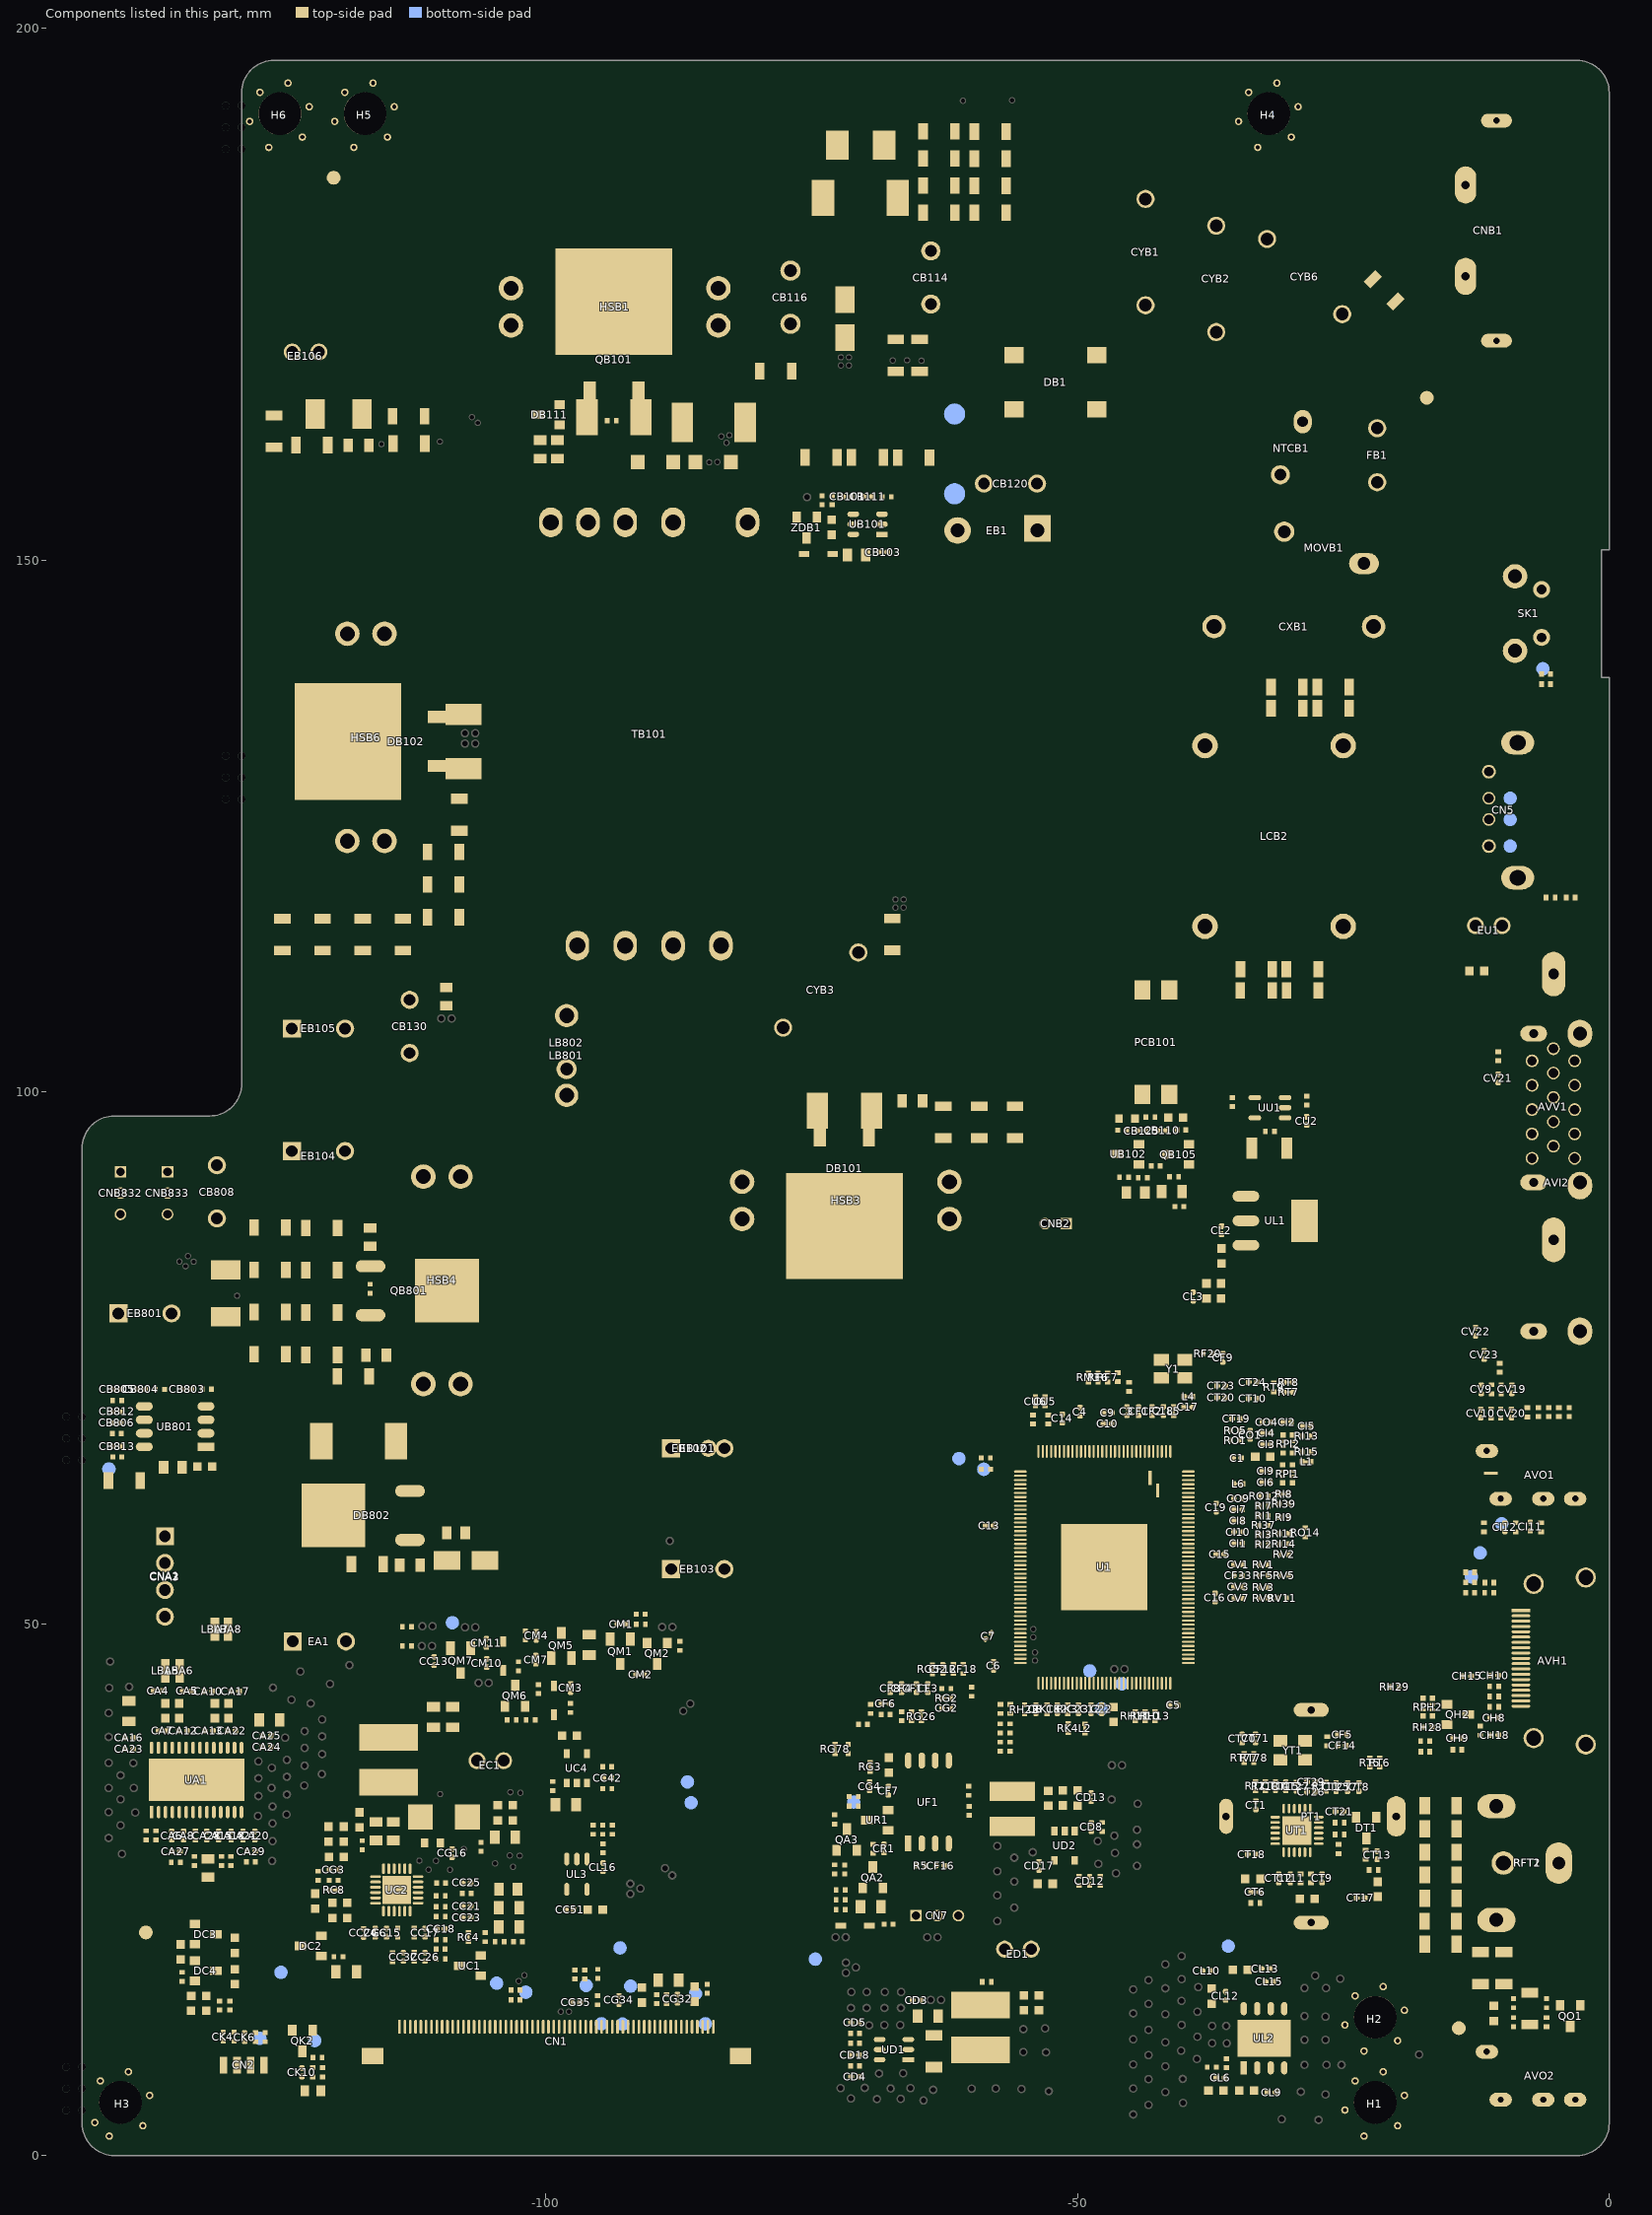
[diagram p0: the components of this part, seen from the top]
# Altium PCB MISC86383-9.PcbDoc (part 6 of 18)
Units mm, origin at the board's own origin, x right, y up, seen from the top; angles counter-clockwise.
Board outline 143.6 x 197 mm, 2 copper layers (TopLayer, BottomLayer), stack 1.571 mm thick; 743 components, 401 nets, 2996 pads, 1077 vias.
Unrouted connection lines stored in the file: 4.

## Footprints (in the part's own frame and the unit in brackets; to place one, negate y for a bottom-side part, rotate by r counter-clockwise, add the part's x,y. Pads: shape width x height; smd on the part's side, far side on the other; paste and mask are expansions set on the pad) (continued)
TO-252 [mm] "与TO-223兼容；15.12.29"
  oval 1.143x2.794 smd: 1(-2.3,-3.6) 3(2.3,-3.6)
  rect 6x6 smd paste-10: 2(0,3.6)
  rect 4x2.6 on Top Paste: 4(0,1.957)
  TopLayer pour cut-out: 2.3,-1.932 2.3,-5.055 -2.345,-5.055 -2.64,-4.996 -2.891,-4.829 -3.058,-4.579 -3.117,-4.284 -3.117,-4.284 -2.299,-4.284 -2.299,-2.699 -3.124,-2.699 -3.066,-2.406 -2.899,-2.157 -2.65,-1.99 -2.356,-1.932 -2.356,-1.932
  silkscreen extent -3.4,-1.34 3.4,7.01, body extent -3.4,-4.15 3.4,6.05, height 2.5
TO-252-GDS [mm] "SC08440  IRLR024N"
  rect 6x6 smd: D(0,0)
  oval 1.143x2.794 smd: G(-2.3,-7.2) S(2.3,-7.2)
  silkscreen extent -3.4,-5.64 3.4,3.4, body extent -3.4,-7.75 3.4,2.45, height 2.5
TP [mm] "TEST POINT   (不带paste  1.27mm 直径）"
  round 1.27 smd paste-1.27: 1(0,0)
TP-TDT [mm] "电源放电测试点，间隔7.5mm"
  round 2 smd paste-2: 1(-3.75,0) 2(3.75,0)
  silkscreen extent -5.75,-2 5.75,2
TP_BL [mm] "TEST POINT,专用背光测试点"
  round 1.27 smd paste-1.27: 1(0,0)
  silkscreen extent -6.4,-0.97 0.95,0.96
TSOT23-6 [mm] "MP65151DJ[MPS]/MP1470"
  rect 1.1x0.5 smd: 1(-1.35,0.95)
  oval 1.1x0.5 smd: 2(-1.35,0) 3(-1.35,-0.95) 4(1.35,-0.95) 5(1.35,0) 6(1.35,0.95)
  silkscreen extent -1.99,-1.5 0.85,2.51, body extent -0.85,-1.5 0.85,1.5, height 1
USB-HD-30 [mm] "广业，USB-20161027-0011，17.07.27"
  oval 2.4x3.3 on Top Overlay: 0(-6.35,8.11) 0(6.35,8.11)
  round 1.5 on Top Overlay: 0(-3.37,10.81) 3(3.63,10.81)
  round 1.3 hole 0.9: 1(-3.37,10.81) 4(3.63,10.81)
  round 1.4 on Top Overlay: 1(-0.87,10.81) 2(1.13,10.81)
  round 1.2 hole 0.9: 2(-0.87,10.81) 3(1.13,10.81)
  oval 2.2x3.1 / inner oval 2.2x3.1 / far side oval 2.9x3.8 hole 1.5 slot 2.4 at 90 deg: 5(6.35,8.11) 6(-6.35,8.11)
  KeepOutLayer pour cut-out: -3.063,12.516 -3.825,12.38 -4.475,11.958 -4.911,11.318 -5.064,10.559 -5.064,10.559 -4.765,9.743 -4.118,9.161 -3.275,8.95 -3.275,8.95 1.967,8.95 2.407,9.037 2.781,9.287 3.03,9.66 3.118,10.101 3.118,10.101 3.118,11.085 3.009,11.632 2.699,12.097 2.234,12.407 1.686,12.516 1.686,12.516
  silkscreen extent -6.65,-0.06 6.65,12, body extent -7.4,-2 7.4,11.9, height 9.4
VR(13*5)-V-7.5 [mm] "为勤,VARISTOR,17.01.04修改为椭圆孔;160105更新椭圆孔 //0424_2019在顶层加整块白油,(12/9/2019按规格书修改高度，从17.5mm改为15.5mm)"
  oval 2.8x2 hole 1.2 slot 2 at 0 deg: 1(3.75,-1.5)
  round 1.9 hole 1.2: 2(-3.75,1.5)
  round 2.1 on Top Overlay: 2(-3.75,1.5)
  oval 3x2.2 on Top Overlay: 2(3.75,-1.5)
  silkscreen extent -6.65,-2.5 6.44,2.5, body extent -6.5,-2.75 6.5,2.75, height 15.5
XTAL-S-3 [mm] "三星（SQ3D03200D2IBA）晶振"
  rect 1.4x1.1 smd: 1(-1.1,-0.85) 2(1.1,-0.85) 3(1.1,0.85) 4(-1.1,0.85)
  silkscreen extent -2.37,-1.91 1.65,1.3, body extent -1.65,-1.3 1.65,1.3, height 0.8
XTAL-S-10 [mm] "铜陵晶威特；SMD3225"
  rect 1.3x1.1 smd: 1(-1.15,-0.9) 2(1.15,-0.9) 3(1.15,0.9) 4(-1.15,0.9)
  silkscreen extent -1.66,-2.5 1.65,1.3, body extent -1.65,-1.3 1.65,1.31, height 0.8

## Part data
AVH1: library part XXX.XXX.0001809-D, "HDMI jack,HDMI Jack,H,Block up,SMD,51U019S-313HFN-E-R-F,FREEPORT-D"
AVI2: library part XXX.XXX.0003577-DLMI, "RCA jack,RCA Jack,AV3,H,Red、White、Yellow,CH5.5,D14,Seal,DIP,RC075-F03L3BY-L,YUQIU-DLMI"
AVO1 AVO2: library part "耳机端子,Earphone Jack,H,Φ3.6,CH5.5,Black,DIP-DLMI"
AVV1: library part WLHD-051A-DLMI-DB15, "CN-DB15-horizontal-#-#-#"
BB101 BB802: library part 004.004.0001046-D, "Ferrite bead,BEAD,50ohm,3.0×4.0,9A,SMD,TP,SMB-302540-K5B-L1,SOLDIER-D"
BB801: library part 004.004.0000346-D, "Ferrite bead,BEAD,80ohm,0805,4000mA,SMD,TP,UPZ2012D800-4R0TF,Sunlord-D"
C1: library part 2.2uF-0402-X5R-±20%-6.3V-D
C2 C11 CA31 CA32 CC50 CD10 CD14 CD15 CD16 CF10 CG31 CL1 CL4 CL5 CL7 CL8 CL11 CL14 CO77 CU1: library part 10uF-0603-X5R-±20%-6.3V-D
C3 C4 C5 C9 C10 C12 C22 CC51 CO1 CO4 CR1 CT6: library part 1uF-0402-X5R-±20%-6.3V-D
C6 C7 C8 C13 C14 C15 C16 C17 C18 C19 C23 CA23 CA24 CA28 CC13 CF7 CF16 CG2 CG3 CG4 CH8 CH9 CH18 CI3 CI4 CI6 CI9 CK4 CK10 CL2 CL3 CM1 CM2 CM4 CT1 CT9 CT11 CT18 CT20 CT21 CT23 CT25 CT27 CU2: library part 0.1uF-0402-Y5V-+80%-20%-16V-D
CA4 CA5 CA10 CA16 CA17 CA25 CA27 CA29 CB103 CF3 CF4 CF6 CF8 CF11 CF12 CI11 CI12: library part 1000pF-0402-X7R-±10%-50V-D
CA6 CA8 CA20 CA21: library part 0.22uF-0402-X5R-±10%-16V-D
CA7 CA12 CA13 CA22: library part 0.22uF-0402-Y5V-+80%-20%-16V-D
CA15 CA18 CC15 CC17 CC18 CG6 CH15: library part 1uF-0402-X5R-±20%-16V-D
CA36 CC29 CC30 CC43 CM5: library part 10uF-0805-X5R-±20%-16V-D
CB101 CB111 CB803 CB813 CI2 CI5 CO9: library part 100pF-0402-NPO-±5%-50V-D
CB102 CB109 CC5 CC7 CC9 CC10 CC11 CC27 CC31 CC34 CC38 CG14 CG33: library part 0.1uF-0603-X7R-±10%-50V-D, "CAP"
CB110 CB125 CB806: library part 1000pF-0402-X7R-±10%-50V-D, "CAP"
CB113: library part 220PF-0805-NPO-±10%-200V-D, "CAP"
CB114: library part C242G472J20A201(编带/法拉)-DAI, "CAP"
CB115: library part 0.1uF-0805-X7R-±10%-50V-D, "CAP"
CB116: library part 004.003.0001889-DHAI, "Ceramic capacitor,CAP CD,1KV,100pF,±5%,SL,OK,5.0mm,DIP,TP,TDK-DHAI"
CB117: library part 1000pF-0805-NPO-±10%-200V-D, "CAP"
CB118: library part "陶瓷电容,CAP MC,1KV,4700pF,±10%,X7R,1206,SMD,TP,ISND-D"
CB120 CB808: library part 004.003.0001665, "Ceramic capacitor,CAP CD,1KV,4700pF,±20%,Y5U,K,5.0mm,DIP,TP,Walsin-DHAI"
CB130: library part 004.003.0000886, "Ceramic capacitor,CAP CD,1KV,4700pF,±20%,Y5U,P,5.0mm,DIP,TP,TongHao-DHAI"
CB801: library part 1uf-0603-X7R-±10%-25V-D
CB804: library part 4700pF-0402-X7R-±10%-50V-D
CB805: library part 0.1uF-0402-X7R-±10%-16V-D
CB809 CB810: library part 004.003.0001392, "Ceramic capacitor,CAP MC,500V,47pF,±5%,NPO,0805,SMD,TP,WALSIN-D"
CB812: library part 0.033uF-0402-X7R-±10%-16V-D
CC1 CC2 CC8 CC12 CC19: library part 22uF-0805-X5R-±20%-6.3V-D
CC4 CC20 CC33 CG22 CG28: library part 1uF-0603-X5R-±10%-50V-D
CC21: library part 1500pF-0402-X7R-±10%-50V-D, "CAP"
CC23 CC24 CC42 CD13 CD17 CG32 CG34 CG35 CL6 CL9 CL10 CL12 CL13 CL15 CL16 CM3: library part 0.1uF-0402-X5R-±20%-16V-D
CC25 CC26 CC32 CH10: library part 33pF-0402-NPO-±5%-50V-D
CD1: library part 004.003.0000514-D, "Ceramic capacitor,CAP MC,16V,10uF,±10%,X5R,1206,SMD,TP-D"
CD2: library part 004.003.0000386-D, "Ceramic capacitor,CAP MC,16V,10uF,±20%,X5R,0805,SMD,TP-D"
CD3 CD4 CD8 CD18: library part 004.003.0000403-D, "Ceramic capacitor,CAP MC,16V,0.1uF,±20%,X5R,0402,SMD,TP-D"
CD5: library part 004.003.0000558-D, "Ceramic capacitor,CAP MC,50V,470pF,±5%,NPO,0402,SMD,TP-D"
CD7 CD9: library part 004.003.0000394-D, "Ceramic capacitor,CAP MC,10V,10uF,±20%,X5R,0603,SMD,TP-D"
CD12: library part 3300pF-0402-X7R-±10%-50V-D
CF1 CF2: library part 004.003.0000527-D, "Ceramic capacitor,CAP MC,50V,18pF,±5%,NPO,0402,SMD,TP-D"
CF5 CU5 CU6 L1 L2 L4 L5 L6 RC4 RC8 RG2 RG3 RG26 RG52 RG78 RI8 RT7 RT8 RT77 RT78: library part 0ohm-0402-PCB-D, "0ohm-0402-PCB-D"
CF9 CF14 CV9 CV10 CV19 CV20 CV21 CV22 CV23: library part 30pF-0402-NPO-±5%-50V-D
CF33 CI1 CI7 CI8 CI10 CV1 CV3 CV7: library part 0.047uF-0402-X7R-±10%-16V-D
CG16: library part 68pF-0402-NPO-±5%-50V-D
CK2: library part 0.01uF-0402-X7R-±10%-50V-D
CK6: library part 10pF-0402-NPO-±5%-50V-D
CM7 CT12 CT19: library part 0.022uF-0402-X7R-±10%-16V-D
CM10: library part 0.022uF-0402-X7R-±10%-50V-D
CM11: library part 004.003.0000398-D, "Ceramic capacitor,CAP MC,16V,0.22uF,±20%,X5R,0402,SMD,TP-D"
CN1: library part XXX.XXX.0004396-D, "FFC connector,FFC connector,60Pin,D0.5,Bottom,lock,SMD,0.5-22-60PBX-P,XFE-D"
CN2: library part 红外接收三极管,Phototransistor,NPN,6.8×3×3.2mm,SMD,HS75438D,VISHAY-D
CN5: library part PKG-003212/P000071027, "USB jack,USB2.0,H,Single,Block up,DIP,U250FD004S1549BY-DLMI"
CN7: library part 3PIN-2.0-D-H-G-带扣-DHMI
CNA1: library part 4PIN-2.54-D-H-G-DHMI
CNA2: library part XXX.XXX.0001836-DLMI, "Connector socket,connect jack,4PIN,D2.50,L,SNAP,STEP,Fool-proofing,Nature,L=3.0mm,DIP,AMA-DLMI"
CNA3: library part 4PIN-2.54-D-H-G-带扣-B-DHMI
CNB1: library part "连接插座,connect jack,2Pin,D8.6,L,SNAP,Fool-proofing,Black,L=4.0mm,DIP,YQ-DLMI", "AC插座-八字侧出"
CNB2: library part XXX.XXX.0001753, "Connector socket,connect jack,2Pin,D2.0,D,L=2.8mm,DIP,AMA-DHMI"
CNB832: library part XXX.XXX.0001754, "Connector socket,connect jack,3Pin,D2.0,D,L=2.8mm,DIP,AMA-DHMI"
CNB833: library part XXX.XXX.0001725-DLMI, "Connector socket,connect jack,3Pin,D2.0,L,SNAP,STEP,Nature,L=2.8mm,DIP,AMA-DLMI"
CT2 CT5: library part 004.003.0000383-D, "Ceramic capacitor,CAP MC,6.3V,10uF,±20%,X5R,0603,SMD,TP-D"
CT7 CT8: library part 004.003.0000530-D, "Ceramic capacitor,CAP MC,50V,22pF,±5%,NPO,0402,SMD,TP-D"
CT10 CT24 CT70 CT71: library part 56pF-0402-NPO-±5%-50V-D
CT13: library part 1.8pF-0402-NPO-±0.25pF-50V-D
CT14 CT15: library part 8pF-0402-NPO-±5%-50V-D
CT17: library part 120pF-0402-NPO-±5%-50V-D
CT26: library part 330pF-0402-NPO-±5%-50V-D
CT29: library part 6800pF-0402-X7R-±10%-50V-D
CT40: library part 4700pF-1206-X7R-±10%-1000V-D
CT41 CT42 CT43 CT44 CT45 CT46 CT47 CT48: library part 1000pF-1206-X7R-±20%-2000V-D
CXB1: library part "X电容,CAP X2,MP,275VAC,0.47uF,±10%,S,15mm-Mini,PC,DIP,BM-DHMI", "CAP"
CYB1 CYB2 CYB3 CYB6: library part "Y电容,CAP Y1,CD,470pF,400VAC,±20%,KS,10mm,Y5U,DIP,Walsin-DHMI", "Y1 capacitor"
DA1 DM1 DM3: library part 1N4148WS-D
DAS1: library part DOLBY_AS2
DB1: library part 004.005.0000860-D, "Bridge rectifier,DIO BRD,3A,800V,YBS,SMD,YBS3010A,YJ-D"
DB101: library part 004.005.0000140-D, "Rectifier diode,DIO SI D1,10A,150V,TO-263,SMD,MBRB10150CT,GOOD-ARK-D"
DB102: library part 004.005.0000473, "Rectifier diode,DIO FRD D1,10A,400V,TO-263,SMD,MURB1040S,GOOD-ARK-D"
DB104 DB804: library part M7(WEJ)-D, "Diode"
DB106 DB801: library part 004.005.0000432-D, "Rectifier diode,DIO SI S,3A,1000V,SMC,SMD,GS3M,GULF-D"
DB107: library part 004.005.0000138-D, "Rectifier diode,DIO FRD S,3A,600V,SMB,SMD,MURS360BT3G,ON-D"
DB109 DB110: library part "整流二极管,DIO FRD S,1.2A,800V,eSGA,SMD,R12K,GOOD-ARK-D"
DB111: library part LBAV70LT1G(LRC)-D, "Diode"
DB112: library part BAV21WS-D, "Diode"
DB802: library part 004.005.0000494-D, "Schottky diode,DIO SBD D1,10A,150V,TO-252,SMD,MBRD10150CT,GOOD-ARK-D"
DC1: library part SK34A-SMA-F-D
DC2 DC3 DC4: library part BAT54S-D
DH2 DH3 DH6 DH7 DI1 DI2 DI3 DI5 DK1 DK2 DO1 DO2 DO3 DR1 DT2 DT3 DU1 DU2 DU3 DU4 DV1 DV2 DV3 DV4 DV5 DV6 DV7 DV8: library part AVLC18S02003-D
DK6: library part 004.005.0000435, "TVS diode,DIO ESD,0.5pF,25V,0402 DFN,SMD,AZ5325-01F.R7G,Amazing-D"
DK20: library part WEJT61RC-871-红色-D
DT1: library part BAV99-BR-D
EA1: library part 470uF-25V-±20%-10×12-105℃-YE-编带-F=5.0(Elite)-DHAI, "Electrolytic"
EB1: library part 004.003.0000164-DLMI, "Aluminium electrolytic capacitor,CAP AL,400V,120uF,±20%,KM,BK,7.5mm,18×35.5,DIP,CapXon-DLMI"
EB101 EB103: library part 470uF-25V-±20%-10×12.5-105℃-GF-编带-F=5.0(CapXon)-DHAI, "Electrolytic"
EB102: library part 270uF-16V-±20%-8×11-105℃-RP-短脚-F=3.5(Elite)-DHMI, "CAP"
EB104 EB105: library part 100uF-63V-±20%-10×12.5-105℃-GF-编带-F=5.0(CapXon)-DHAI, "Electrolytic"
EB106: library part 10uF-50V-±20%-5×11-105℃-GH-编带-F=2.5(CapXon)-DHAI, "Electrolytic"
EB801: library part 47uF-100V-±20%-10×12-105℃-EV-编带-F=5.0(Elite)-DHAI, "Electrolytic"
EC1: library part 100uF-35V-±20%-6.3×11-105℃-KF-编带-F=2.5(CapXon)-DHAI, "Electrolytic"
ED1 EU1: library part 470uF-10V-±20%-6.3×11-105℃-黑底白字-编带-F=2.5-XF-DHAI, "Electrolytic"
EVA1 EVA2 EVA3 EVA4 EVA5 EVA6: library part 7×7×3mm-C-4305防火泡棉-黑色-DLMI, "EVA"
F2: library part 5R1ohm-0402-±5%-1/16W-D
FB1: library part 004.026.0000010-DHMI, "Slow-blow fuse,FUSE T,P,3.15A,250VAC,8.5×4.0×8mm,DIP,TP,Walter-DHMI"
FU1: library part 004.026.0000039-D, "Self-resetting fuse,FUSE PTC,1.1A,6V,1206,SMD,TP,TLC-D"
GD1 GD2 GD3: library part 7.00×8.35mm-尼龙-白色-WQM-DHMI, "Mylar stud"
GL1 GL2 GL3 GL4 GL5: library part 005.002.0000011, "Silicone,0.2g,general,60,white,SLD-8854W,XY-DHMI"
H1 H2 H3 H4 H5 H6: library part "Location hole-D"
HS1: library part 18.8×13.8×5-本色-THD-HS, "SMD heat sink"
HS2: library part 004.040.0008928-D, "Heat sink,15.0×15.0×5.0mm,AL1060H-24,black,high-emissivity paint,stamped with bend,no press-fit legs,YT-D"
HSB1 HSB3 HSB4 HSB6: library part 004.040.0006600-DHMI, "Heat sink,17.5×14.5×0.5mm,red copper sheet,bright tin plated,natural,four pins,WT-DHMI"
LB801: library part SYDR1212-L003-EDL-DHMI, "I-type inductor"
LB802: library part 差模电感,Inductor,DR12×14,68uH,0.45,20Ts,H13.5MAX,SYDR1214-L068uA,DIP,Soldier-DHMI, "I-type inductor"
LBA1 LBA2 LBA3 LBA4: library part 004.004.0000104-D, "Multilayer inductor,HF Inductor,220nH,±5%,0603,SMD,SWI0603F-R22J,Tai-tech-D"
LBA5 LBA6 LBA7 LBA8: library part 0ohm-0603-PCB-D, "0ohm-0603-PCB-D"
LC1: library part SCD54TL-6R8M-D
LCB2: library part 004.004.0002597-DHMI, "Common-mode choke,Common Choke,UC1614,10.5mH±10%,0.15×1.0mm,48Ts,H14.0MAX,SYUC16-L10.5mA,DIP,CH-DHMI"
LD1: library part 004.004.0000017-D, "Power inductor,Power Inductor,4.7uH,±20%,2.8A,0.35×1P,DR5.8×4.5,SMD,SCD54TL-4R7M,Soldier-D"
LD2: library part SLN43T-6R8M-D
LF1: library part MGHB1005S102T-LF-D
LT1: library part SDCL1005C68NJTDF(68nH-0402±5%-C)-D
LT2 LT6 LT8: library part 1Kohm-0402-±25%-D
LT3: library part 2.2nH-0402-±0.3nH-1/4-D
LT9: library part SDCL1005CR33JTDF-D
LT10: library part SDCL1608CR22JT(F)-D
LT11: library part SDCL1005CR27JTDF(顺络)-D
LT12: library part GZ1005U121CTF(120ohm-500mA)-D
M1 M2 M3 M4: library part MARK-D
ML1: library part MALAY
MOVB1: library part TVR10561KSW(为勤)-DHMI, "Varistor"
NTCB1: library part SCK102R55AMBY502(短脚/为勤)-DHMI, "Thermistor"
PCB101: library part LTV-817S-TA-B(光宝)-DMI, "Optocoupler"
PCB101及周围贴片器件 RB101,102,143,144电阻附近 UB101及周围贴片器件 UB801及周围贴片器件: library part 0.05g-导热硅脂, "Thermal grease"
PT1: library part 20.3×16.3×6-LHD(带封口)-DMI
PWM_REF: library part TEST
QA2: library part 3CG3906M-D, "Q-PNP-#-#-#"
QA3 QH2 QK2: library part MMBT3904(f≥350MHz)-D-NPN, "Q-NPN-#-#-#"
QB101: library part 004.007.0000227-D, "MOSFET,NMOS,13.7A,650V,0.22ohm@ID=6.9A@VGS=10V,D2PAK,TK14G65W,TOSHIBA-D"
QB105 QM2 QM6 QO1: library part LMBT3904LT1G-D-NPN, "Q-NPN-#-#-#"
QB801: library part AOD4454(AOS)-D, "N Channel Single MOSFET"
QM1: library part WPM2341A-3/TR-D
QM5: library part WPM3407C-3/TR-D
QM7: library part 004.007.0000286-D, "MOSFET,PMOS,-4.7A,-20V,70mohm@ID=-4.7A@VGS=-4.5V,SOT23-LC,LPB3443LT1G,LRC-D"
R5 RB804 RC24 RG7 RG12 RH10 RH11 RK20 RL50 RL51 RM3 RM4 RO6 RT2 RT18 RV4 RV14: library part 10Kohm-0402-±5%-1/16W-D
RA1 RA8 RK13 RO9 RV6 RV10 RV18 RV19 RV20 RV21 RV22 RV23: library part 100ohm-0402-±5%-1/16W-D
RA2 RA15 RI10: library part GND
RA3 RC1: library part 10ohm-0805-±5%-1/8W-D
RA4 RC13 RC18 RC27 RM7: library part 47Kohm-0402-±5%-1/16W-D
RA5 RA21: library part 180ohm-0402-±5%-1/16W-D
RA10 RH14 RK3 RK16 RK21 RO10 RR1 RR5 RR6: library part 1Kohm-0402-±5%-1/16W-D
RA11: library part 12Kohm-0402-±5%-1/16W-D
RA12: library part 9K1ohm-0402-±5%-1/16W-D
RA14 RC19 RC20 RC23 RC33 RG5 RG6 RG25 RG39 RG40 RG41 RG42 RG43 RG44 RG46 RG48 RG59 RG62 RH1 RH2 RI11 RI13 RI14 RI15 RO14: library part 0ohm-0402-±5%-1/16W-D
RA16: library part 8K2ohm-0402-±5%-1/16W-D
RA18 RA19: library part 33Kohm-0402-±5%-1/16W-D
RA31: library part 470Kohm-0402-±5%-1/16W-D
RA38 RC10 RG49 RM2 RR2: library part 100Kohm-0402-±5%-1/16W-D
RB1 RB2 RB3 RB4 RB160: library part 1M2ohm-1206-±5%-1/4W-D, "RES"
RB101 RB102: library part 330Kohm-1206-±5%-1/4W-D, "RES"
RB103: library part 6K8ohm-0402-±1%-1/16W-D
RB104: library part 27Kohm-0402-±1%-1/16W-D
RB105: library part 510ohm-0402-±1%-1/16W-D
RB106: library part 68ohm-0805-±5%-1/8W-D
RB107 RB807: library part 20ohm-0805-±5%-1/8W-D, "RES"
RB109 RB133 RB182 RB808: library part 10Kohm-0402-±1%-1/16W-D
RB110 RB116 RB117 RB118 RB119 RB810 RB812: library part 10ohm-1206-±5%-1/4W-D, "RES"
RB112 RB140: library part 51Kohm-0805-±1%-1/8W-D, "RES"
RB114 RB115: library part 4R7ohm-1206-±1%-1/4W-D, "RES"
RB124 RB125 RB126 RB127 RB162 RB163 RB164 RB165: library part 68ohm-1206-±5%-1/4W-D, "RES"
RB128 RB129: library part 47ohm-1206-±5%-1/4W-D, "RES"
RB130: library part 20ohm-1206-±5%-1/4W-D
RB131: library part 2Kohm-0603-±5%-1/10W-D
RB132 RB806: library part 1Kohm-0402-±1%-1/16W-D
RB134: library part 4K7ohm-0402-±1%-1/16W-D, "RES"
RB135: library part 18Kohm-0402-±1%-1/16W-D, "RES"
RB141 RB142 RB143 RB144 RB145: library part 2Mohm-1206-±5%-1/4W-D, "RES"
RB148: library part 004.002.0001050, "Thick film resistor,RES,2W,0.22ohm,±5%,2512,SMD-D"
RB150 RB151 RB152 RB153 RB154 RB155 RB156 RB157: library part 100Kohm-1206-±5%-1/4W-D, "RES"
RB158: library part 3Kohm-0402-±1%-1/16W-D
RB180: library part 20Kohm-0402-±1%-1/16W-D
RB181: library part 1Kohm-0805-±1%-1/8W-D
RB183 RK4 RK6 RU45: library part 4K7ohm-0402-±1%-1/16W-D
RB803 RC35: library part 9K1ohm-0402-±1%-1/16W-D
RB805: library part 100ohm-0402-±5%-1/16W-D, "RES"
RB813: library part 100ohm-0402-±1%-1/16W-D
RB814: library part 004.002.0001261, "Thick film resistor,RES,1/4W,510Kohm,±1%,1206-Auto,SMD-D"
RB816: library part 33ohm-0805-±5%-1/8W-D
RB818 RB819 RB820 RB821: library part 0R3ohm-1206-±5%-1/4W-D
RB837 RB838: library part 1R5ohm-1206-±1%-1/4W-D, "RES"
RB839: library part 2R2ohm-1206-±1%-1/4W-D, "RES"
RB840: library part 1R6ohm-1206-±1%-1/4W-D, "RES"
RC2: library part 12Kohm-0402-±1%-1/16W-D
RC3: library part 1K2ohm-0402-±1%-1/16W-D
RC12: library part 56Kohm-0402-±1%-1/16W-D
RC14: library part 4R7ohm-0402-±5%-1/16W-D
RC15: library part 121Kohm-0402-±1%-1/16W-D
RC31 RG16: library part 16Kohm-0402-±1%-1/16W-D
RC32: library part 10ohm-0402-±1%-1/16W-D
RC36 RGV1: library part 10ohm-0402-±5%-1/16W-D
RD1 RD7: library part 004.002.0000579-D, "Thick film resistor,RES,1/16W,100Kohm,±5%,0402,SMD-D"
RD3: library part 004.002.0000806-D, "Thick film resistor,RES,1/16W,60.4Kohm,±1%,0402,SMD-D"
RD5: library part 004.002.0000573-D, "Thick film resistor,RES,1/16W,10.5Kohm,±1%,0402,SMD-D"
RD8: library part 004.002.0000593-D, "Thick film resistor,RES,1/16W,13Kohm,±1%,0402,SMD-D"
RD9: library part 004.002.0000588-D, "Thick film resistor,RES,1/16W,12Kohm,±1%,0402,SMD-D"
RF5 RI7 RI37: library part 68ohm-0402-±5%-1/16W-D
RF6 RF7 RF13 RF14 RF18 RK15 RK18 RU4 RV12 RV13: library part 4K7ohm-0402-±5%-1/16W-D
RF20 RH13 RH28 RH29 RT9: library part 220ohm-0402-±5%-1/16W-D
RFT1: library part "RF头,RF JACK,H,F,T14.5,CH6.3,without pipe,12.4×13.2×7.7mm,DIP,LHD-DLMI", "T-F-6.3mm-#-#"
RFT2: library part "RF头,RF JACK,H,IEC,T14.5,CH6.3,12.4×13.2×7.7mm,DIP,LHD-020组件,LHD-DLMI", "T-IEC-6.3mm-#-#"
RG8: library part 470Kohm-0402-±1%-1/16W-D
RG9: library part 100Kohm-0402-±1%-1/16W-D
RG13: library part 39Kohm-0402-±1%-1/16W-D, "RES"
RG14: library part 6K2ohm-0402-±1%-1/16W-D
RG15: library part 18Kohm-0402-±1%-1/16W-D
RG21: library part 62Kohm-0402-±1%-1/16W-D
RG22: library part 7K5ohm-0402-±1%-1/16W-D
RG58 RG63: library part 1Kohm-0805-±5%-1/8W-D
RG60 RG61 RT5 RT6 RV1 RV3 RV9: library part 33ohm-0402-±5%-1/16W-D
RG82: library part 10ohm-0603-±5%-1/10W-D
RH22: library part 300Kohm-0402-±5%-1/16W-D
RI1 RI2 RL4: library part 150ohm-0402-±1%-1/16W-D
RI3 RI9 RI39 RO12 RV2 RV5 RV11: library part 75ohm-0402-±5%-1/16W-D
RK1: library part 22ohm-0402-±5%-1/16W-D
RL3 RL7: library part 004.002.0000689-D, "Thick film resistor,RES,1/16W,4.7Kohm,±5%,0402,SMD-D"
RL5: library part 91ohm-0402-±1%-1/16W-D
RM1 RM5 RM6 RM8: library part 4k7ohm-0402-±5%-1/16W-D
RM10: library part 2K2ohm-0402-±5%-1/16W-D
RM12: library part 004.002.0000578-D, "Thick film resistor,RES,1/16W,100Kohm,±1%,0402,SMD-D"
RO1 RO5: library part 510ohm-0402-±5%-1/16W-D
RO2: library part 100ohm-1206-±5%-1/4W-D, "RES"
RPH2 RPI1 RPI2: library part 4*100ohm-0402-±5%-1/16W-D
RT11: library part 1K8ohm-0402-±5%-1/16W-D
SK1: library part "轻触开关,Tact Switch,160±50gf,7.0×10.3×7.0mm,DIP,KFC-A06-E-4-7.5/4(R),YK-DLMI"
TB101: library part 004.004.0002512-DLMI, "Transformer,Transformer,EQ2612,230uH,0.2×2P,25Ts,H14.5MAX,SYEQ2613Z-T012033A(BLACK),DIP,SQ-DLMI"
TP-TDT: library part TEST, "TEST"
U1: library part "TV主芯片,IC Main Chip,MSD3553NBCT-005X,32bit,Single-Core,EpLQFP156,SMD,Mstar-D"
UA1: library part "音频功放,IC Audio AMP,Class D,2×9W@13V@8ohm,HTSSOP28,SMD,TPA3136D2,TI-D"
UB101: library part LD7537RGL(通嘉)-D, "IC"
UB102: library part AZ431AN-ATRE1(BCD)-D, "SMD 431"
UB801: library part OB3350CPA(OB)-D, "IC"
UC1: library part TL431G-AE2-R(UTC)-D
UC2: library part G5517-D
UC4: library part "运算放大器,IC OP Amplifier,1 channel,18MHz,TSOT23-5,SMD,ANX7003AAK,ANAX"
UD1: library part 004.010.0001184-D, "DC-DC IC,IC DC-DC,Syn,2A,18V,600KHz,SOT23-6,SMD,TMI3252T,TOLL-D"
UD2: library part "DC-DCоƬ,IC DCDC,Syn,1.2A,7.0V,1.5MHz,SOT23-5,SMD,LC2127CB5TR,Leadchip-D"
UF1: library part "SPI FLASH оƬ,IC SPI FLASH,64Mb,SOIC8,SMD,GD25Q64CSIG,GigaDevice-D"
UL1: library part LC1117CLTR18-D
UL2: library part LC1118-D
UL3: library part 004.010.0000105-D, "LDO IC,IC LDO,0.5A,3.3V,10V,SOT23-5,SMD,LC1458CB5TR33,LEADCHIP-D"
UR1: library part SGM810-SXN3L-D
UT1: library part R840-D
UU1: library part 004.010.0000334-D, "Current limit switch,IC OCP,0.4-2A adj,5.5V,H,SOT23-5,SMD,SY6280AAAC,SILERGY-D"
Y1: library part 32MHz-±10PPM-12PF-SMD3225-JWT-D
YT1: library part 004.009.0000056, "Passive standard-package crystal oscillator,SPXO,24MHz,±20ppm,16pF,3.2×2.5,SMD,SMD3225 24.000MHZ,JWT-D"
ZDB1: library part LBZX84C24LT1G(LRC)-D, "Diode"
用于U1上: library part Φ12mm×12mm-黑色-125度(UL认证)-D